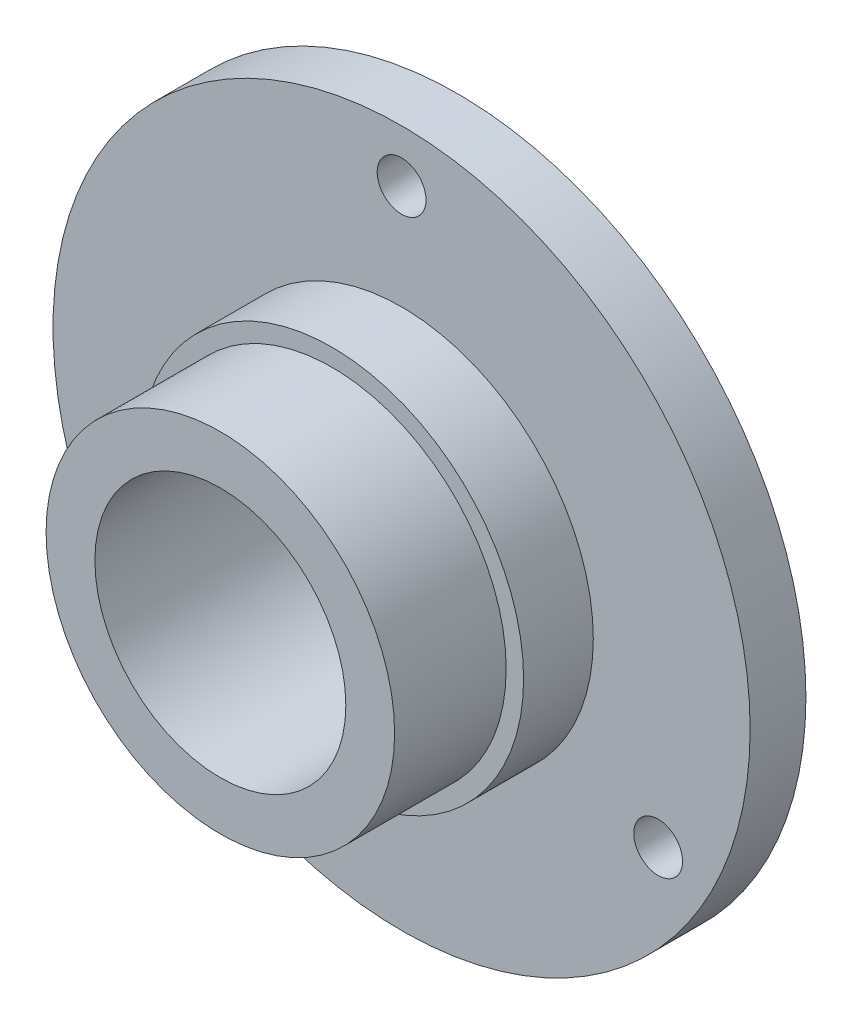
SolidWorks part; units mm, degrees
material "普通碳钢"
ref_plane "Front Plane" through (0, 0, 0) normal (0, 0, 1) x (1, 0, 0)
ref_plane "Top Plane" through (0, 0, 0) normal (0, 1, 0) x (1, 0, 0)
ref_plane "Right Plane" through (0, 0, 0) normal (1, 0, 0) x (0, 0, -1)
sketch "Sketch1" plane through (0, 0, 0) normal (0, 0, 1) x (1, 0, 0)
  line L0 (0, 42.5) -> (0, 0) construction
  line L1 (0, 0) -> (-36.8061, -21.25) construction
  line L2 (0, 0) -> (36.8061, -21.25) construction
  circle A0 centre (0, 0) radius 50
  circle A2 centre (0, 0) radius 42.5 construction
  circle A3 centre (0, 42.5) radius 3.5
  circle A4 centre (-36.8061, -21.25) radius 3.5
  circle A5 centre (36.8061, -21.25) radius 3.5
  circle A6 centre (0, 0) radius 18
  dimension "D1" = 100
  dimension "D2" = 85
  dimension "D3" = 7
  dimension "D6" = 36
  dimension "D4" = 120
  dimension "D5" = 120
extrude "Boss-Extrude1" add sketch "Sketch1" along normal blind 8
sketch "Sketch2" plane through (0, 0, 8) normal (0, 0, 1) x (1, 0, 0)
  circle A0 centre (0, 0) radius 27.5
  circle A1 centre (0, 0) radius 18
  dimension "D1" = 55
  dimension "D2" = 36
extrude "Boss-Extrude2" add sketch "Sketch2" along normal blind 10
sketch "Sketch3" plane through (0, 0, 18) normal (0, 0, 1) x (1, 0, 0)
  circle A0 centre (0, 0) radius 25
  circle A1 centre (0, 0) radius 18
  dimension "D1" = 50
  dimension "D2" = 36
extrude "Boss-Extrude3" add sketch "Sketch3" along normal blind 16
